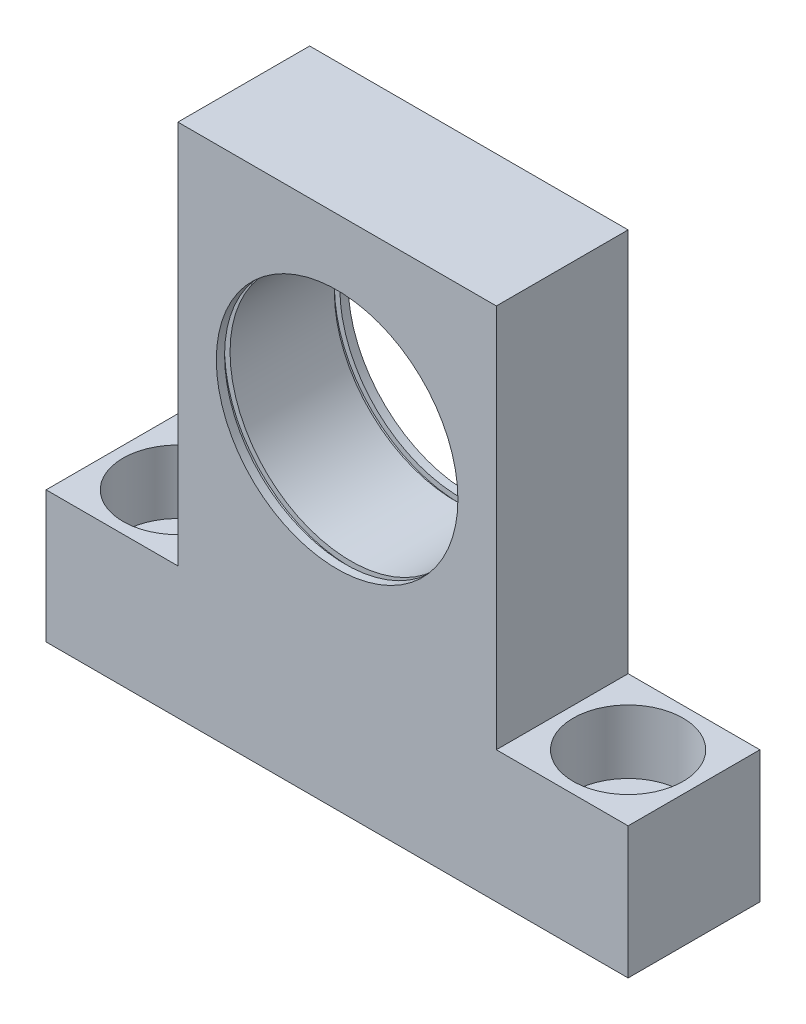
from build123d import *

# Parameters (mm, degrees)
SKETCH_1_R          = 11
EXTRUDE_1_DEPTH     = 12
SKETCH_2_R          = 2.75
CUT_EXTRUDE_1_DEPTH = 53.135542299
SKETCH_3_R          = 5
CUT_EXTRUDE_2_DEPTH = 5.8
SKETCH_4_R          = 11.5
CUT_EXTRUDE_3_DEPTH = 0.25
SKETCH_5_R          = 11.5
CUT_EXTRUDE_4_DEPTH = 0.25


with BuildPart() as part:
    # 草图1 → 凸台-拉伸1 (new body)
    with BuildSketch(Plane.XY):
        Polygon((-16.269702277, -16.03765324), (36.730297723, -16.03765324), (36.730297723, -4.03765324), (24.730297723, -4.03765324), (24.730297723, 30.96234676), (-4.269702277, 30.96234676), (-4.269702277, -4.03765324), (-16.269702277, -4.03765324), align=None)
        with Locations((10.230297723, 13.96234676)):
            Circle(SKETCH_1_R, mode=Mode.SUBTRACT)
    extrude(amount=EXTRUDE_1_DEPTH)

    # 草图2 → 切除-拉伸1 (cut, through all)
    with BuildSketch(Plane(origin=(0, -4.03765324, 0), x_dir=(1, 0, 0), z_dir=(0, 1, 0))):
        with Locations(Location((-10.269702277, -6, 0), (0, 0, 180))):
            Circle(SKETCH_2_R)
        with Locations(Location((30.730297723, -6, 0), (0, 0, 180))):
            Circle(SKETCH_2_R)
    extrude(amount=-CUT_EXTRUDE_1_DEPTH, mode=Mode.SUBTRACT)

    # 草图3 → 切除-拉伸2 (cut)
    with BuildSketch(Plane(origin=(0, -4.03765324, 0), x_dir=(1, 0, 0), z_dir=(0, 1, 0))):
        with Locations(Location((-10.269702277, -6, 0), (0, 0, 180))):
            Circle(SKETCH_3_R)
        with Locations(Location((30.730297723, -6, 0), (0, 0, 180))):
            Circle(SKETCH_3_R)
    extrude(amount=-CUT_EXTRUDE_2_DEPTH, mode=Mode.SUBTRACT)

    # 草图4 → 切除-拉伸3 (cut, symmetric)
    with BuildSketch(Plane.XY.offset(11)):
        with Locations((10.230297723, 13.96234676)):
            Circle(SKETCH_4_R)
    extrude(amount=CUT_EXTRUDE_3_DEPTH, both=True, mode=Mode.SUBTRACT)

    # 草图5 → 切除-拉伸4 (cut, symmetric)
    with BuildSketch(Plane(origin=(0, 0, 1), x_dir=(-1, 0, 0), z_dir=(0, 0, -1))):
        with Locations(Location((-10.230297723, 13.96234676, 0), (0, 0, 180))):
            Circle(SKETCH_5_R)
    extrude(amount=CUT_EXTRUDE_4_DEPTH, both=True, mode=Mode.SUBTRACT)


solid = part.part
